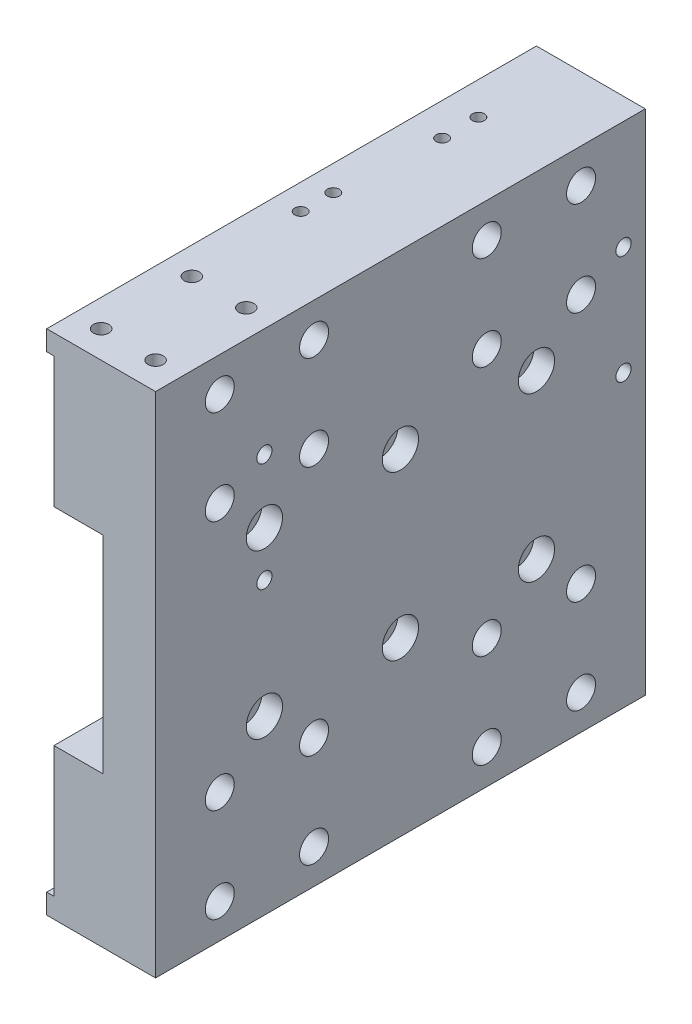
from build123d import *

# Parameters (mm, degrees)
SKETCH1_W                                            = 135
SKETCH1_H                                            = 140
BOSS_EXTRUDE1_DEPTH                                  = 30
SKETCH2_W                                            = 15.5
SKETCH2_H                                            = 57
CUT_EXTRUDE1_DEPTH                                   = 156
SKETCH3_W                                            = 135
SKETCH3_H                                            = 129
CUT_EXTRUDE2_DEPTH                                   = 2
M4_TAPPED_HOLE1_D                                    = 3.3
M4_TAPPED_HOLE1_DEPTH                                = 10.1
M4_TAPPED_HOLE1_TIP                                  = 0.991420021
M5_TAPPED_HOLE1_D                                    = 4.2
M5_TAPPED_HOLE1_DEPTH                                = 12.4
M5_TAPPED_HOLE1_TIP                                  = 1.2618073
F_5_0MM_DOWEL_HOLE1_D                                = 5
F_5_0MM_DOWEL_HOLE1_DEPTH                            = 8
F_5_0MM_DOWEL_HOLE1_TIP                              = 1.502151548
M5_TAPPED_HOLE2_D                                    = 4.2
M5_TAPPED_HOLE2_DEPTH                                = 12.4
M5_TAPPED_HOLE2_TIP                                  = 1.2618073
CBORE_FOR_M4_HEXAGON_SOCKET_HEAD_CAP_SCR_D           = 4.5
CBORE_FOR_M4_HEXAGON_SOCKET_HEAD_CAP_SCR_CBORE_D     = 8
CBORE_FOR_M4_HEXAGON_SOCKET_HEAD_CAP_SCR_CBORE_DEPTH = 23
CBORE_FOR_M5_HEXAGON_SOCKET_HEAD_CAP_SCR_D           = 5.5
CBORE_FOR_M5_HEXAGON_SOCKET_HEAD_CAP_SCR_CBORE_D     = 10
CBORE_FOR_M5_HEXAGON_SOCKET_HEAD_CAP_SCR_CBORE_DEPTH = 5.7
LPATTERN1_COUNT                                      = 2
LPATTERN1_PITCH                                      = 37.5
LPATTERN1_COL_COUNT                                  = 2
LPATTERN1_COL_PITCH                                  = 37.5
M5_TAPPED_HOLE3_D                                    = 4.2
M5_TAPPED_HOLE3_DEPTH                                = 12.4
M5_TAPPED_HOLE3_TIP                                  = 1.2618073
M4_TAPPED_HOLE2_D                                    = 3.3
M4_TAPPED_HOLE2_DEPTH                                = 10.1
M4_TAPPED_HOLE2_TIP                                  = 0.991420021


with BuildPart() as part:
    # Sketch1 → Boss-Extrude1 (new body)
    with BuildSketch(Plane(origin=(0, 0, 0), x_dir=(0, 0, -1), z_dir=(1, 0, 0))):
        Rectangle(SKETCH1_W, SKETCH1_H)
    extrude(amount=BOSS_EXTRUDE1_DEPTH)

    # Sketch2 → Cut-Extrude1 (cut, through all)
    with BuildSketch(Plane(origin=(0, 0, -67.5), x_dir=(-1, 0, 0), z_dir=(0, 0, -1))):
        with Locations((-7.75, 0)):
            Rectangle(SKETCH2_W, SKETCH2_H)
    extrude(amount=-CUT_EXTRUDE1_DEPTH, mode=Mode.SUBTRACT)

    # Sketch3 → Cut-Extrude2 (cut)
    with BuildSketch(Plane.ZY):
        Rectangle(SKETCH3_W, SKETCH3_H)
    extrude(amount=-CUT_EXTRUDE2_DEPTH, mode=Mode.SUBTRACT)

    # M4 Tapped Hole1
    with Locations(Plane(origin=(0, 70, 0), x_dir=(1, 0, 0), z_dir=(0, 1, 0))):
        with Locations((7, 4.5), (7, -4.5)):
            Hole(M4_TAPPED_HOLE1_D / 2, depth=M4_TAPPED_HOLE1_DEPTH)
            with Locations((0, 0, -(M4_TAPPED_HOLE1_DEPTH + M4_TAPPED_HOLE1_TIP / 2))):  # 118° drill point
                Cone(0, M4_TAPPED_HOLE1_D / 2, M4_TAPPED_HOLE1_TIP, mode=Mode.SUBTRACT)

    # M5 Tapped Hole1
    with Locations(Plane(origin=(0, -70, 0), x_dir=(-1, 0, 0), z_dir=(0, -1, 0))):
        with Locations((-24, 33.75), (-6, 33.75), (-24, -33.75), (-6, -33.75)):
            Hole(M5_TAPPED_HOLE1_D / 2, depth=M5_TAPPED_HOLE1_DEPTH)
            with Locations((0, 0, -(M5_TAPPED_HOLE1_DEPTH + M5_TAPPED_HOLE1_TIP / 2))):  # 118° drill point
                Cone(0, M5_TAPPED_HOLE1_D / 2, M5_TAPPED_HOLE1_TIP, mode=Mode.SUBTRACT)

    # Ø5.0mm dowel hole1
    with Locations(Plane(origin=(0, -70, 0), x_dir=(-1, 0, 0), z_dir=(0, -1, 0))):
        with Locations((-15, 33.75), (-15, -33.75)):
            Hole(F_5_0MM_DOWEL_HOLE1_D / 2, depth=F_5_0MM_DOWEL_HOLE1_DEPTH)
            with Locations((0, 0, -(F_5_0MM_DOWEL_HOLE1_DEPTH + F_5_0MM_DOWEL_HOLE1_TIP / 2))):  # 118° drill point
                Cone(0, F_5_0MM_DOWEL_HOLE1_D / 2, F_5_0MM_DOWEL_HOLE1_TIP, mode=Mode.SUBTRACT)

    # M5 Tapped Hole2
    with Locations(Plane(origin=(30, 0, 0), x_dir=(0, 0, -1), z_dir=(1, 0, 0))):
        with Locations((-37.5, 40), (-37.5, 10), (61.5, 40), (61.5, 10)):
            Hole(M5_TAPPED_HOLE2_D / 2, depth=M5_TAPPED_HOLE2_DEPTH)
            with Locations((0, 0, -(M5_TAPPED_HOLE2_DEPTH + M5_TAPPED_HOLE2_TIP / 2))):  # 118° drill point
                Cone(0, M5_TAPPED_HOLE2_D / 2, M5_TAPPED_HOLE2_TIP, mode=Mode.SUBTRACT)

    # CBORE for M4 Hexagon socket head cap screws1 (through all)
    with Locations(Plane(origin=(30, 0, 0), x_dir=(0, 0, -1), z_dir=(1, 0, 0))):
        with Locations((-49.8, 60.5), (-23.8, 60.5), (-23.8, 34.5), (-49.8, 34.5), (49.8, 34.5), (23.8, 34.5), (23.8, 60.5), (49.8, 60.5), (49.8, -60.5), (23.8, -60.5), (23.8, -34.5), (49.8, -34.5), (-49.8, -34.5), (-23.8, -34.5), (-23.8, -60.5), (-49.8, -60.5)):
            CounterBoreHole(CBORE_FOR_M4_HEXAGON_SOCKET_HEAD_CAP_SCR_D / 2, CBORE_FOR_M4_HEXAGON_SOCKET_HEAD_CAP_SCR_CBORE_D / 2, CBORE_FOR_M4_HEXAGON_SOCKET_HEAD_CAP_SCR_CBORE_DEPTH)

    # CBORE for M5 Hexagon socket head cap screws1 (through all)
    with Locations(Plane(origin=(30, 0, 0), x_dir=(0, 0, -1), z_dir=(1, 0, 0))):
        with Locations((0, 22.5), (0, -22.5)):
            cbore_for_m5_hexagon_socket_head_cap_scr = CounterBoreHole(CBORE_FOR_M5_HEXAGON_SOCKET_HEAD_CAP_SCR_D / 2, CBORE_FOR_M5_HEXAGON_SOCKET_HEAD_CAP_SCR_CBORE_D / 2, CBORE_FOR_M5_HEXAGON_SOCKET_HEAD_CAP_SCR_CBORE_DEPTH)

    # LPattern1: CBORE for M5 Hexagon socket head cap screws1 ×2
    with Locations(*[(0, 0, i * LPATTERN1_PITCH) for i in range(1, LPATTERN1_COUNT)]):
        add(cbore_for_m5_hexagon_socket_head_cap_scr, mode=Mode.SUBTRACT)

    # LPattern1 col: CBORE for M5 Hexagon socket head cap screws1 ×2
    with Locations(*[(0, 0, -i * LPATTERN1_COL_PITCH) for i in range(1, LPATTERN1_COL_COUNT)]):
        add(cbore_for_m5_hexagon_socket_head_cap_scr, mode=Mode.SUBTRACT)

    # M5 Tapped Hole3
    with Locations(Plane(origin=(0, 70, 0), x_dir=(1, 0, 0), z_dir=(0, 1, 0))):
        with Locations((7.5, -60), (22.5, -60), (22.5, -35), (7.5, -35)):
            Hole(M5_TAPPED_HOLE3_D / 2, depth=M5_TAPPED_HOLE3_DEPTH)
            with Locations((0, 0, -(M5_TAPPED_HOLE3_DEPTH + M5_TAPPED_HOLE3_TIP / 2))):  # 118° drill point
                Cone(0, M5_TAPPED_HOLE3_D / 2, M5_TAPPED_HOLE3_TIP, mode=Mode.SUBTRACT)

    # M4 Tapped Hole2
    with Locations(Plane(origin=(0, 70, 0), x_dir=(1, 0, 0), z_dir=(0, 1, 0))):
        with Locations((9, 42.5), (9, 32.5)):
            Hole(M4_TAPPED_HOLE2_D / 2, depth=M4_TAPPED_HOLE2_DEPTH)
            with Locations((0, 0, -(M4_TAPPED_HOLE2_DEPTH + M4_TAPPED_HOLE2_TIP / 2))):  # 118° drill point
                Cone(0, M4_TAPPED_HOLE2_D / 2, M4_TAPPED_HOLE2_TIP, mode=Mode.SUBTRACT)


solid = part.part
